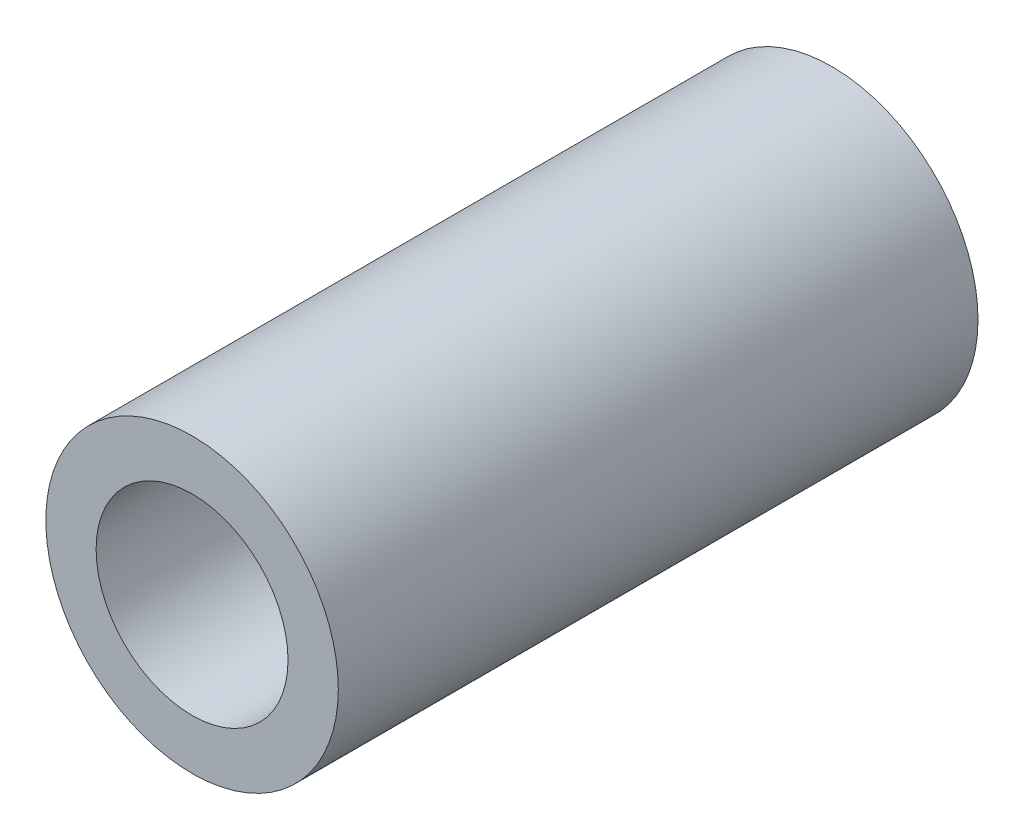
SolidWorks part; units mm, degrees
material "20"
ref_plane "Front Plane" through (0, 0, 0) normal (0, 0, 1) x (1, 0, 0)
ref_plane "Top Plane" through (0, 0, 0) normal (0, 1, 0) x (1, 0, 0)
ref_plane "Right Plane" through (0, 0, 0) normal (1, 0, 0) x (0, 0, -1)
sketch "Sketch1" plane through (0, 0, 0) normal (0, 0, 1) x (1, 0, 0)
  circle A0 centre (0, 0) radius 8
  dimension "D1" = 16
extrude "Boss-Extrude1" add sketch "Sketch1" along normal blind 35
hole_wizard "M12x1.25 Tapped Hole1" positions "Sketch3" profile "Sketch2" tap size "M12x1.25" standard "GB"
sketch "Sketch3" plane through (0, 0, 35) normal (0, 0, 1) x (1, 0, 0)
  point P0 (0, 0)
sketch "Sketch2" plane through (0, 0, 35) normal (1, 0, 0) x (0, -1, 0)
  line L0 (0, 0) -> (0, 38.1545)
  line L1 (0, 38.1545) -> (5.25, 35)
  line L2 (5.25, 35) -> (5.25, 0)
  line L5 (5.25, 0) -> (0, 0)
  line L10 (0, 38.1545) -> (-5.25, 35) construction
  line L11 (0, -6.35) -> (0, 107.95) construction
  dimension "螺纹孔钻头直径" = 10.5
  dimension "螺纹孔钻头深度" = 35
  dimension "导头角度" = 118
cosmetic thread "Cosmetic thread2"
